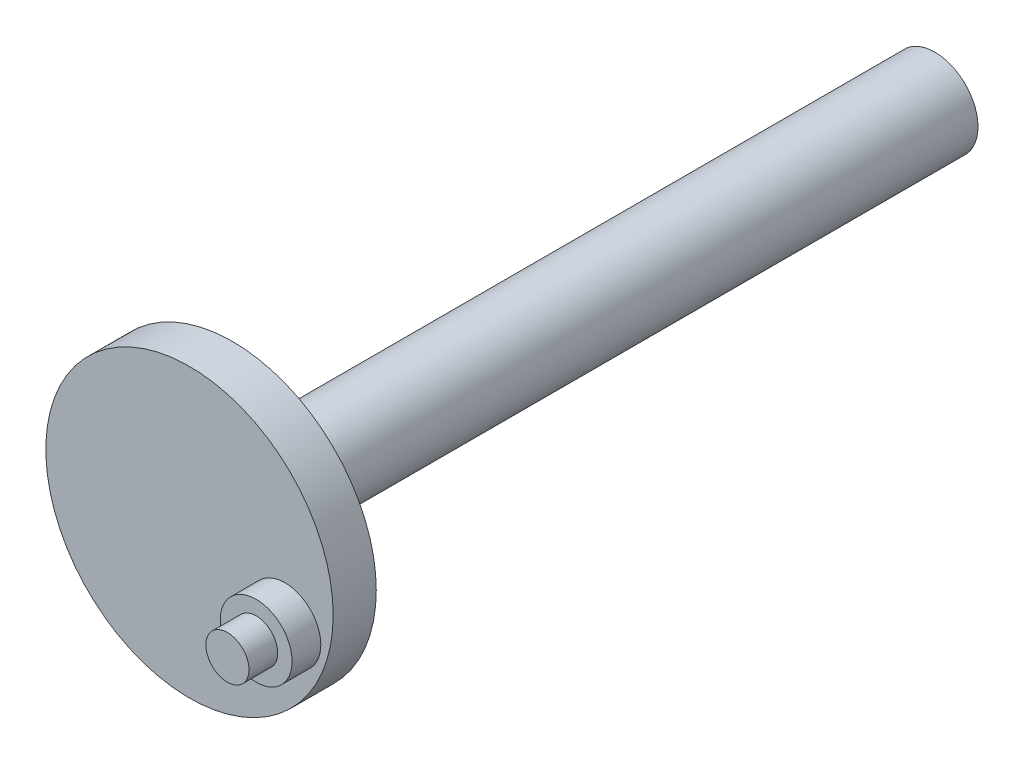
from build123d import *

# Parameters (mm, degrees)
SKETCH1_R           = 10
BOSS_EXTRUDE1_DEPTH = 3
SKETCH2_R           = 2.5
BOSS_EXTRUDE2_DEPTH = 2
SKETCH3_R           = 1.5
BOSS_EXTRUDE3_DEPTH = 2
SKETCH4_R           = 3
BOSS_EXTRUDE4_DEPTH = 50
CUT_EXTRUDE1_START  = -2.12
SKETCH5_R           = 3
CUT_EXTRUDE1_DEPTH  = 2.12
SKETCH6_R           = 3
BOSS_EXTRUDE5_DEPTH = 1


with BuildPart() as part:
    # Sketch1 → Boss-Extrude1 (new body)
    with BuildSketch(Plane.XY):
        with Locations((9.394956339, 17.03797738)):
            Circle(SKETCH1_R)
    extrude(amount=BOSS_EXTRUDE1_DEPTH)

    # Sketch2 → Boss-Extrude2 (add)
    with BuildSketch(Plane.XY.offset(3)):
        with Locations((16.034106962, 14.819491633)):
            Circle(SKETCH2_R)
    extrude(amount=BOSS_EXTRUDE2_DEPTH)

    # Sketch3 → Boss-Extrude3 (add)
    with BuildSketch(Plane.XY.offset(5)):
        with Locations((16.034106962, 14.819491633)):
            Circle(SKETCH3_R)
    extrude(amount=BOSS_EXTRUDE3_DEPTH)

    # Sketch4 → Boss-Extrude4 (add)
    with BuildSketch(Plane(origin=(0, 0, 0), x_dir=(-1, 0, 0), z_dir=(0, 0, -1))):
        with Locations(Location((-9.394956339, 17.03797738, 0), (0, 0, 180))):
            Circle(SKETCH4_R)
    extrude(amount=BOSS_EXTRUDE4_DEPTH)

    # Sketch5 → Cut-Extrude1 (cut)
    with BuildSketch(Plane(origin=(0, 0, -50), x_dir=(-1, 0, 0), z_dir=(0, 0, -1)).offset(CUT_EXTRUDE1_START)):
        with Locations(Location((-9.394956339, 17.03797738, 0), (0, 0, 180))):
            Circle(SKETCH5_R)
    extrude(amount=CUT_EXTRUDE1_DEPTH, mode=Mode.SUBTRACT)

    # Sketch6 → Boss-Extrude5 (add)
    with BuildSketch(Plane(origin=(0, 0, -47.88), x_dir=(-1, 0, 0), z_dir=(0, 0, -1))):
        with Locations(Location((-9.394956339, 17.03797738, 0), (0, 0, 180))):
            Circle(SKETCH6_R)
    extrude(amount=BOSS_EXTRUDE5_DEPTH)


solid = part.part
